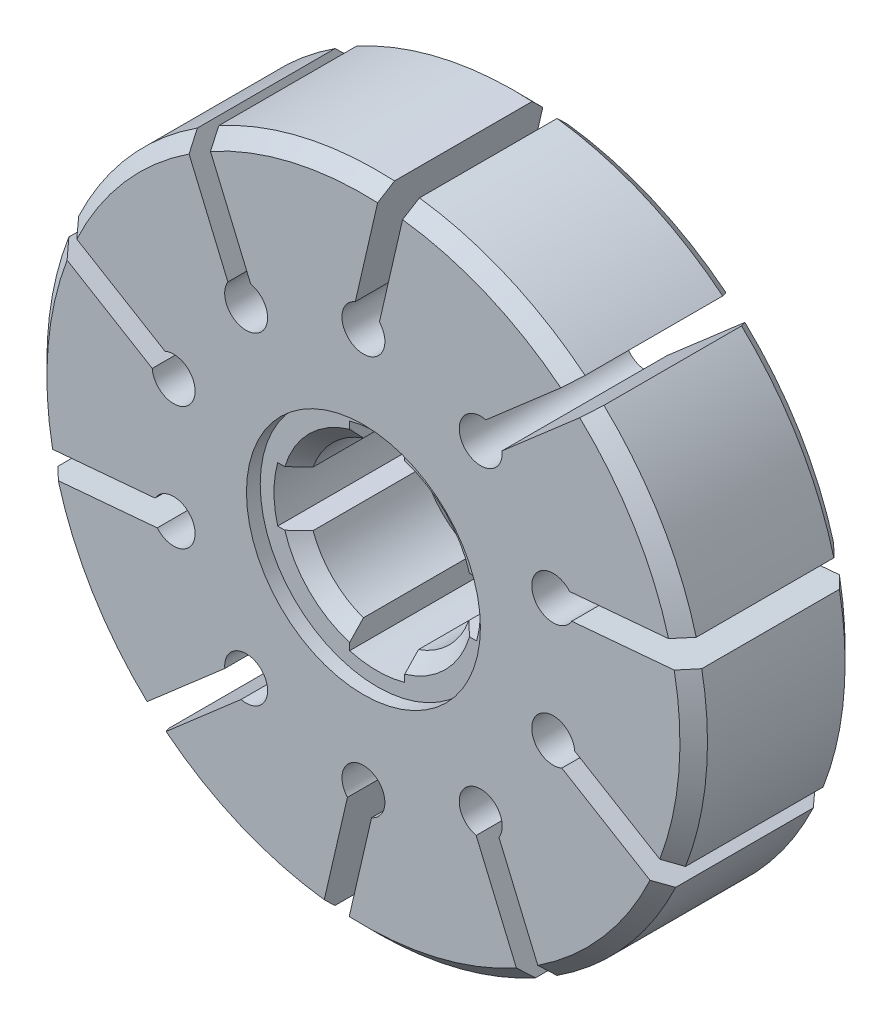
from build123d import *

# Parameters (mm, degrees)
SKETCH_1_R               = 24
EXTRUDE_1_DEPTH          = 12
CHAMFER_1_SIZE           = 1
SKETCH_2_R               = 8.5
CUT_EXTRUDE_1_DEPTH      = 1
CUT_EXTRUDE_START        = -1
SKETCH_3_R               = 8.5
CUT_EXTRUDE_2_DEPTH      = 1
SKETCH_4_R               = 6
CUT_EXTRUDE_3_DEPTH      = 36.67912555
CHAMFER_2_SIZE           = 1
CUT_EXTRUDE_4_DEPTH      = 36.67912555
CUT_EXTRUDE_5_DEPTH      = 37
PATTERN_CIRCULAR_1_COUNT = 10


with BuildPart() as part:
    # 草图1 → 凸台-拉伸1 (new body)
    with BuildSketch(Plane.XY):
        Circle(SKETCH_1_R)
    extrude(amount=EXTRUDE_1_DEPTH)

    # 倒角1
    chamfer_1_edges = [part.edges().sort_by_distance(p)[0] for p in [
        (-24, 0, 0),
        (-24, 0, 12),
    ]]
    chamfer(chamfer_1_edges, length=CHAMFER_1_SIZE)

    # 草图2 → 切除-拉伸1 (cut)
    with BuildSketch(Plane.XY.offset(12)):
        Circle(SKETCH_2_R)
    extrude(amount=-CUT_EXTRUDE_1_DEPTH, mode=Mode.SUBTRACT)

    # 草图3 → 切除-拉伸2 (cut)
    with BuildSketch(Plane(origin=(0, 0, 0), x_dir=(-1, 0, 0), z_dir=(0, 0, -1)).offset(CUT_EXTRUDE_START)):
        with Locations(Location((0, 0, 0), (0, 0, 180))):
            Circle(SKETCH_3_R)
    extrude(amount=CUT_EXTRUDE_2_DEPTH, mode=Mode.SUBTRACT)

    # 草图4 → 切除-拉伸3 (cut, through all)
    with BuildSketch(Plane.XY.offset(11)):
        Circle(SKETCH_4_R)
    extrude(amount=-CUT_EXTRUDE_3_DEPTH, mode=Mode.SUBTRACT)

    # 倒角2
    chamfer_2_edges = [part.edges().sort_by_distance(p)[0] for p in [
        (-6, 0, 1),
        (-6, 0, 11),
    ]]
    chamfer(chamfer_2_edges, length=CHAMFER_2_SIZE)

    # 草图5 → 切除-拉伸4 (cut, through all)
    with BuildSketch(Plane.XY.offset(11)):
        with BuildLine():
            Line((-2, 7.228416147), (-2, 2))
            Line((-2, 2), (-7.228416147, 2))
            ThreePointArc((-7.228416147, 2), (-7.5, 0), (-7.228416147, -2))
            Line((-7.228416147, -2), (-2, -2))
            Line((-2, -2), (-2, -5.656854249))
            Line((-2, -5.656854249), (-2, -7.228416147))
            ThreePointArc((-2, -7.228416147), (0, -7.5), (2, -7.228416147))
            Line((2, -7.228416147), (2, -5.656854249))
            Line((2, -5.656854249), (2, -2))
            Line((2, -2), (7.228416147, -2))
            ThreePointArc((7.228416147, -2), (7.5, 0), (7.228416147, 2))
            Line((7.228416147, 2), (2, 2))
            Line((2, 2), (2, 7.228416147))
            ThreePointArc((2, 7.228416147), (0, 7.5), (-2, 7.228416147))
        make_face()
    extrude(amount=-CUT_EXTRUDE_4_DEPTH, mode=Mode.SUBTRACT)

    # 草图6 → 切除-拉伸5 (cut, through all)
    with BuildSketch(Plane.XY.offset(12)):
        with BuildLine():
            Line((1.163498987, 15.538797459), (3.353568182, 25.02502934))
            Line((3.353568182, 25.02502934), (1.564387139, 25.276975484))
            Line((1.564387139, 25.276975484), (-0.590367129, 15.943709357))
            ThreePointArc((-0.590367129, 15.943709357), (-0.350868128, 12.980223171), (1.163498987, 15.538797459))
        make_face()
    cut_extrude_5 = extrude(amount=-CUT_EXTRUDE_5_DEPTH, mode=Mode.SUBTRACT)

    # 阵列(圆周)1: 切除-拉伸5 ×10 about axis
    pattern_circular_1_axis = Axis((0, 0, 0), (0, 0, 1))
    for i in range(1, PATTERN_CIRCULAR_1_COUNT):
        add(cut_extrude_5.rotate(pattern_circular_1_axis, i * 360 / PATTERN_CIRCULAR_1_COUNT), mode=Mode.SUBTRACT)


solid = part.part
